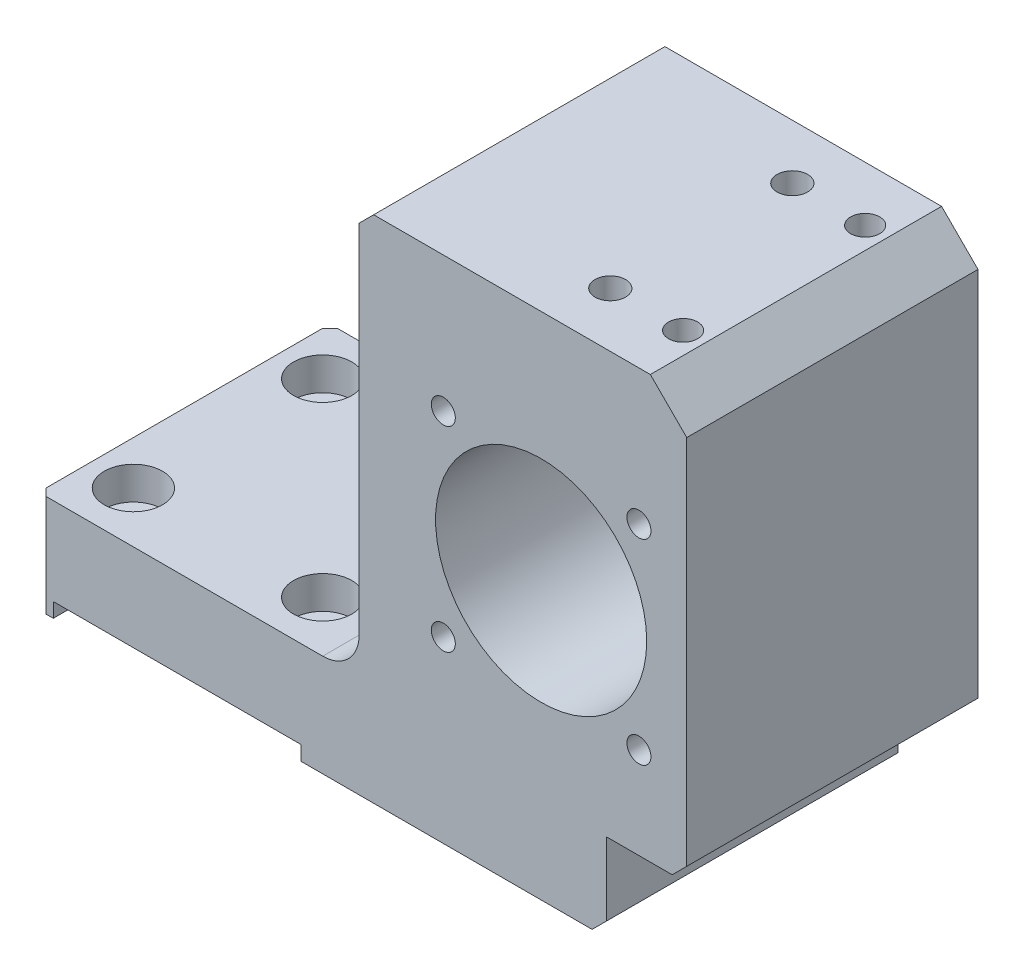
SolidWorks part; units mm, degrees
material "A7075"
ref_plane "Front Plane" through (0, 0, 0) normal (0, 0, 1) x (1, 0, 0)
ref_plane "Top Plane" through (0, 0, 0) normal (0, 1, 0) x (1, 0, 0)
ref_plane "Right Plane" through (0, 0, 0) normal (1, 0, 0) x (0, 0, -1)
sketch "Sketch1" plane through (0, 0, 0) normal (0, 0, 1) x (1, 0, 0)
  line L0 (0, 0) -> (89, 0)
  line L1 (89, 0) -> (89, 70)
  line L2 (89, 70) -> (44, 70)
  line L3 (44, 70) -> (44, 14)
  line L4 (44, 14) -> (0, 14)
  line L5 (0, 14) -> (0, 0)
  circle A0 centre (69, 38) radius 14.5
  dimension "D1" = 29
  dimension "D7" = 20
  dimension "D2" = 45
  dimension "D3" = 38
  dimension "D4" = 14
  dimension "D5" = 70
  dimension "D6" = 89
extrude "Boss-Extrude1" add sketch "Sketch1" along normal mid plane 40
hole_wizard "Ø4.5 (4.5) Diameter Hole1" positions "Sketch3" profile "Sketch4" hole size "Ø4.5" standard "Gb" end condition through all
sketch "Sketch3" plane through (0, 0, 0) normal (0, -1, 0) x (-1, 0, 0)
  line L0 (0, -20) -> (0, 20) construction
  point P0 (-32, 13)
  point P2 (-6, 13)
  point P4 (-6, -13)
  point P6 (-32, -13)
  dimension "D1" = 26
  dimension "D2" = 26
  dimension "D3" = 13
  dimension "D4" = 6
sketch "Sketch4" plane through (32, 0, -13) normal (1, 0, 0) x (0, 0, -1)
  line L0 (0, 0) -> (0, 70)
  line L1 (0, 70) -> (2.25, 70)
  line L2 (2.25, 70) -> (2.25, 0)
  line L5 (2.25, 0) -> (0, 0)
  line L11 (0, -6.35) -> (0, 107.95) construction
  dimension "通孔孔直径" = 4.5
  dimension "通孔孔深度" = 70
sketch "Sketch5" plane through (0, 0, 0) normal (0, -1, 0) x (1, 0, 0)
  line L0 (0, 20) -> (89, 20) construction
  line L1 (2, 20) -> (36, 20)
  line L2 (2, 20) -> (2, -20)
  line L3 (2, -20) -> (36, -20)
  line L4 (36, 20) -> (36, -20)
  line L5 (0, -20) -> (89, -20) construction
  circle A0 centre (6, 13) radius 2.25 construction
  dimension "D1" = 34
  dimension "D2" = 4
extrude "Cut-Extrude1" cut sketch "Sketch5" against normal blind 2
hole_wizard "M4 Tapped Hole1" positions "Sketch7" profile "Sketch6" tap size "M4" standard "Gb"
sketch "Sketch7" plane through (0, 0, 20) normal (0, 0, 1) x (1, 0, 0)
  line L0 (82.435, 24.565) -> (69, 38) construction
  line L1 (69, 38) -> (82.435, 51.435) construction
  line L4 (69, 38) -> (55.565, 51.435) construction
  line L7 (69, 38) -> (69, 57) construction
  circle A0 centre (69, 38) radius 19 construction
  point P0 (55.565, 51.435)
  point P2 (82.435, 51.435)
  point P4 (55.565, 24.565)
  point P6 (82.435, 24.565)
  dimension "D3" = 38
  dimension "D1" = 45
  dimension "D2" = 90
sketch "Sketch6" plane through (55.565, 51.435, 20) normal (1, 0, 0) x (0, -1, 0)
  line L0 (0, 0) -> (0, 11.0914)
  line L1 (0, 11.0914) -> (1.65, 10.1)
  line L2 (1.65, 10.1) -> (1.65, 0)
  line L5 (1.65, 0) -> (0, 0)
  line L10 (0, 11.0914) -> (-1.65, 10.1) construction
  line L11 (0, -6.35) -> (0, 107.95) construction
  dimension "螺纹孔钻头直径" = 3.3
  dimension "螺纹孔钻头深度" = 10.1
  dimension "导头角度" = 118
cosmetic thread "Cosmetic Thread1" parameters "D1"=8, "D2"=4
cosmetic thread "Cosmetic Thread2" parameters "D1"=8, "D2"=4
cosmetic thread "Cosmetic Thread3" parameters "D1"=8, "D2"=4
cosmetic thread "Cosmetic Thread4" parameters "D1"=8, "D2"=4
hole_wizard "M5 Tapped Hole1" positions "Sketch9" profile "Sketch8" tap size "M5" standard "Gb"
sketch "Sketch9" plane through (0, 70, 0) normal (0, 1, 0) x (-1, 0, 0)
  line L0 (-44, 20) -> (-44, -20) construction
  point P0 (-71, -12.5)
  point P2 (-71, 12.5)
  dimension "D1" = 25
  dimension "D2" = 12.5
  dimension "D3" = 27
sketch "Sketch8" plane through (71, 70, -12.5) normal (1, 0, 0) x (0, 0, 1)
  line L0 (0, 0) -> (0, 15.2618)
  line L1 (0, 15.2618) -> (2.1, 14)
  line L2 (2.1, 14) -> (2.1, 0)
  line L5 (2.1, 0) -> (0, 0)
  line L10 (0, 15.2618) -> (-2.1, 14) construction
  line L11 (0, -6.35) -> (0, 107.95) construction
  dimension "螺纹孔钻头直径" = 4.2
  dimension "螺纹孔钻头深度" = 14
  dimension "导头角度" = 118
cosmetic thread "Cosmetic Thread5" parameters "D1"=10, "D2"=5
cosmetic thread "Cosmetic Thread6" parameters "D1"=10, "D2"=5
hole_wizard "Ø4.0 (4) Diameter Hole1" positions "Sketch11" profile "Sketch10" hole size "Ø4.0" standard "Gb"
sketch "Sketch11" plane through (0, 70, 0) normal (0, 1, 0) x (-1, 0, 0)
  line L0 (-81, 12.5) -> (-71, 12.5) construction
  line L3 (-71, -12.5) -> (-81, -12.5) construction
  point P0 (-81, 12.5)
  point P2 (-81, -12.5)
  dimension "D1" = 10
sketch "Sketch10" plane through (81, 70, 12.5) normal (1, 0, 0) x (0, 0, 1)
  line L0 (0, 0) -> (0, 13.2017)
  line L1 (0, 13.2017) -> (2, 12)
  line L2 (2, 12) -> (2, 0)
  line L5 (2, 0) -> (0, 0)
  line L10 (0, 13.2017) -> (-2, 12) construction
  line L11 (0, -6.35) -> (0, 107.95) construction
  dimension "孔直径" = 4
  dimension "孔深度" = 12
  dimension "导头角度" = 118
sketch "Sketch12" plane through (0, 0, 20) normal (0, 0, 1) x (1, 0, 0)
  line L1 (89, 0) -> (78, 0)
  line L2 (89, 0) -> (89, 12)
  line L3 (89, 12) -> (78, 12)
  line L4 (78, 0) -> (78, 12)
  dimension "D1" = 11
  dimension "D2" = 12
extrude "Cut-Extrude2" cut sketch "Sketch12" against normal through all
hole_wizard "M3 Tapped Hole1" positions "Sketch14" profile "Sketch13" tap size "M3" standard "Gb"
sketch "Sketch14" plane through (78, 0, 0) normal (1, 0, 0) x (0, 0, -1)
  line L0 (0, 0) -> (0, 6) construction
  point P0 (-10, 6)
  point P2 (0, 6)
  point P4 (10, 6)
  dimension "D1" = 6
  dimension "D2" = 10
  dimension "D3" = 10
sketch "Sketch13" plane through (78, 6, 10) normal (0, 1, 0) x (0, 0, -1)
  line L0 (0, 0) -> (0, 9.2511)
  line L1 (0, 9.2511) -> (1.25, 8.5)
  line L2 (1.25, 8.5) -> (1.25, 0)
  line L5 (1.25, 0) -> (0, 0)
  line L10 (0, 9.2511) -> (-1.25, 8.5) construction
  line L11 (0, -6.35) -> (0, 107.95) construction
  dimension "螺纹孔钻头直径" = 2.5
  dimension "螺纹孔钻头深度" = 8.5
  dimension "导头角度" = 118
cosmetic thread "Cosmetic Thread7" parameters "D1"=6, "D2"=3
cosmetic thread "Cosmetic Thread8" parameters "D1"=6, "D2"=3
cosmetic thread "Cosmetic Thread9" parameters "D1"=6, "D2"=3
chamfer "Chamfer1" distance 5 angle 45 1 edges at (89, 70, 0)
chamfer "Chamfer2" distance 2 angle 45 3 edges at (78, 0, 0) (89, 12, 0) (44, 70, 0)
sketch "Sketch15" plane through (0, 14, 0) normal (0, 1, 0) x (1, 0, 0)
  circle A0 centre (6, 13) radius 4
  circle A1 centre (32, 13) radius 4
  circle A2 centre (32, -13) radius 4
  circle A3 centre (6, -13) radius 4
  dimension "D1" = 8
extrude "Cut-Extrude3" cut sketch "Sketch15" against normal blind 4.5
fillet "Fillet1" radius 5 1 edges at (44, 14, 0)
chamfer "Chamfer3" distance 1 angle 45 2 edges at (0, 7, -20) (0, 7, 20)
